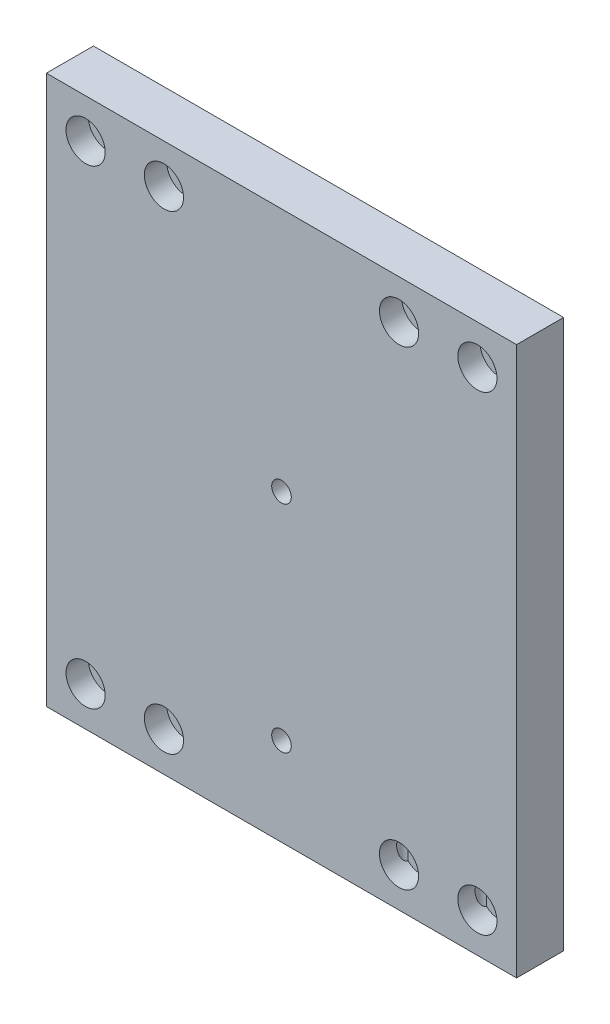
from build123d import *

# Parameters (mm, degrees)
SKETCH_1_W                  = 120
SKETCH_1_H                  = 140
EXTRUDE_1_DEPTH             = 6
HOLE_WIZARD_M6_1_D          = 5
HOLE_WIZARD_M6_1_DEPTH      = 15
HOLE_WIZARD_M6_1_TIP        = 1.502151548
HOLE_WIZARD_1_D             = 5.5
HOLE_WIZARD_1_DEPTH         = 15
HOLE_WIZARD_1_CBORE_D       = 10
HOLE_WIZARD_1_CBORE_DEPTH   = 5.7
HOLE_WIZARD_1_TIP           = 1.652366702
SKETCH_5_R                  = 2.5
CUT_EXTRUDE_1_DEPTH         = 6
HOLE_WIZARD_M4_2_AT_2_COUNT = 2
HOLE_WIZARD_M4_2_AT_2_PITCH = 20


with BuildPart() as part:
    # 草图1 → 凸台-拉伸1 (new, symmetric)
    with BuildSketch(Plane.XY):
        Rectangle(SKETCH_1_W, SKETCH_1_H)
    extrude(amount=EXTRUDE_1_DEPTH, both=True)

    # M6 螺纹孔1
    with Locations(Plane(origin=(0, -47.5, 6), x_dir=(1, 0, 0), z_dir=(0, 0, 1))):
        with Locations((0, 0), (0, 55)):
            Hole(HOLE_WIZARD_M6_1_D / 2, depth=HOLE_WIZARD_M6_1_DEPTH)
            with Locations((0, 0, -(HOLE_WIZARD_M6_1_DEPTH + HOLE_WIZARD_M6_1_TIP / 2))):  # 118° drill point
                Cone(0, HOLE_WIZARD_M6_1_D / 2, HOLE_WIZARD_M6_1_TIP, mode=Mode.SUBTRACT)

    # 打孔尺寸(%根据)内六角圆柱头螺钉的类型1
    with Locations(Plane(origin=(-50, 60, 6), x_dir=(1, 0, 0), z_dir=(0, 0, 1))):
        with Locations((0, 0), (20, 0), (80, 0), (100, 0), (100, -120), (80, -120), (20, -120), (0, -120)):
            CounterBoreHole(HOLE_WIZARD_1_D / 2, HOLE_WIZARD_1_CBORE_D / 2, HOLE_WIZARD_1_CBORE_DEPTH, depth=HOLE_WIZARD_1_DEPTH)
            with Locations((0, 0, -(HOLE_WIZARD_1_DEPTH + HOLE_WIZARD_1_TIP / 2))):  # 118° drill point
                Cone(0, HOLE_WIZARD_1_D / 2, HOLE_WIZARD_1_TIP, mode=Mode.SUBTRACT)

    # 草图5 → 切除-拉伸1 (cut)
    with BuildSketch(Plane(origin=(0, 0, -6), x_dir=(-1, 0, 0), z_dir=(0, 0, -1))):
        with Locations((0, 60)):
            Circle(SKETCH_5_R)
        with Locations((0, -60)):
            Circle(SKETCH_5_R)
    extrude(amount=-CUT_EXTRUDE_1_DEPTH, mode=Mode.SUBTRACT)

    # 草图11 → M4 螺纹孔2 (revolve, cut)
    with BuildSketch(Plane(origin=(25, -70, 0), x_dir=(0, 0, -1), z_dir=(1, 0, 0))):
        Polygon((0, 0), (0, 11.091420021), (1.65, 10.1), (1.65, 0), align=None)
    hole_wizard_m4_2 = revolve(axis=Axis((25, -76.35, 0), (0, 1, 0)), mode=Mode.SUBTRACT)

    # M4 螺纹孔2 at 2: M4 螺纹孔2 ×2
    with Locations(*[(i * HOLE_WIZARD_M4_2_AT_2_PITCH, 0, 0) for i in range(1, HOLE_WIZARD_M4_2_AT_2_COUNT)]):
        add(hole_wizard_m4_2, mode=Mode.SUBTRACT)

    # 镜向1: M4 螺纹孔2 across plane
    add(hole_wizard_m4_2.mirror(Plane(origin=(0, 0, 0), x_dir=(0, 0, 1), z_dir=(1, 0, 0))), mode=Mode.SUBTRACT)

    # 镜向1 copy 1 sketch → 镜向1 copy 1 (revolve, cut)
    with BuildSketch(Plane(origin=(-45, -70, 0), x_dir=(0, 0, -1), z_dir=(-1, 0, 0))):
        Polygon((0, 0), (0, -11.091420021), (1.65, -10.1), (1.65, 0), align=None)
    revolve(axis=Axis((-45, -76.35, 0), (0, -1, 0)), mode=Mode.SUBTRACT)


solid = part.part
